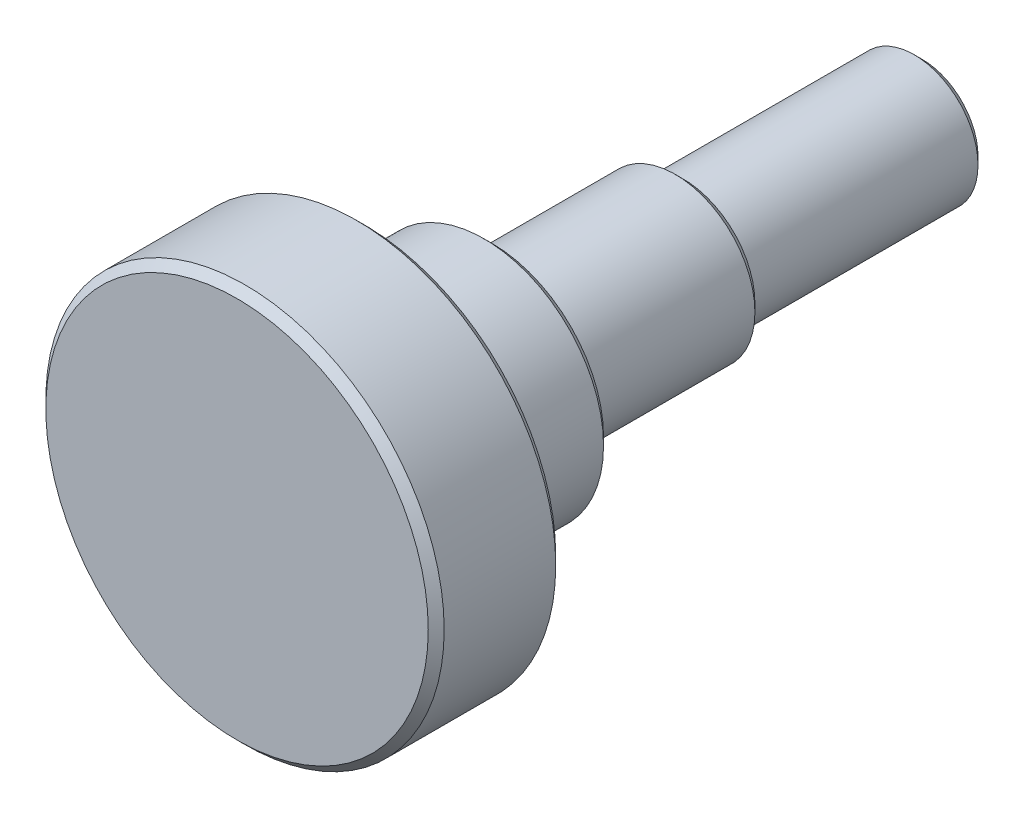
from build123d import *

# Parameters (mm, degrees)
SKETCH1_R           = 4
BOSS_EXTRUDE1_DEPTH = 15
SKETCH2_R           = 5
BOSS_EXTRUDE2_DEPTH = 12
SKETCH3_R           = 7.5
BOSS_EXTRUDE3_DEPTH = 8
SKETCH4_R           = 12.5
BOSS_EXTRUDE4_DEPTH = 8
CHAMFER1_SIZE       = 0.5


with BuildPart() as part:
    # Sketch1 → Boss-Extrude1 (new body)
    with BuildSketch(Plane.XY):
        Circle(SKETCH1_R)
    extrude(amount=BOSS_EXTRUDE1_DEPTH)

    # Sketch2 → Boss-Extrude2 (add)
    with BuildSketch(Plane.XY.offset(15)):
        Circle(SKETCH2_R)
    extrude(amount=BOSS_EXTRUDE2_DEPTH)

    # Sketch3 → Boss-Extrude3 (add)
    with BuildSketch(Plane.XY.offset(27)):
        Circle(SKETCH3_R)
    extrude(amount=BOSS_EXTRUDE3_DEPTH)

    # Sketch4 → Boss-Extrude4 (add)
    with BuildSketch(Plane.XY.offset(35)):
        Circle(SKETCH4_R)
    extrude(amount=BOSS_EXTRUDE4_DEPTH)

    # Chamfer1
    chamfer1_edges = [part.edges().sort_by_distance(p)[0] for p in [
        (-12.5, 0, 35),
        (-12.5, 0, 43),
        (-4, 0, 0),
        (-5, 0, 15),
        (-7.5, 0, 27),
    ]]
    chamfer(chamfer1_edges, length=CHAMFER1_SIZE)


solid = part.part
